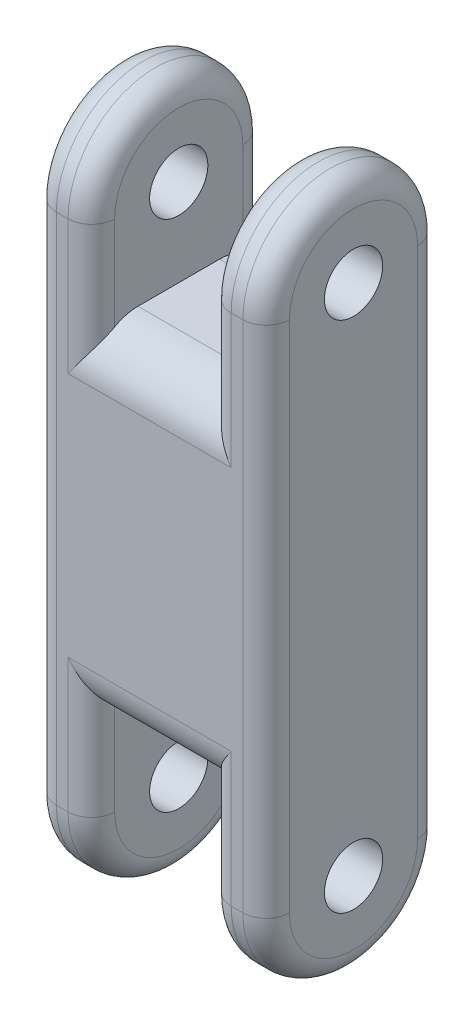
SolidWorks part; units mm, degrees
material "ABS"
ref_plane "Front" through (0, 0, 0) normal (0, 0, 1) x (1, 0, 0)
ref_plane "Top" through (0, 0, 0) normal (0, 1, 0) x (1, 0, 0)
ref_plane "Right" through (0, 0, 0) normal (1, 0, 0) x (0, 0, -1)
sketch "Sketch1" plane through (0, 0, 0) normal (1, 0, 0) x (0, 0, -1)
  line L0 (-4.7625, 0) -> (-4.7625, 27.9908)
  line L1 (4.7625, 27.9908) -> (4.7625, 0)
  arc A0 (-4.7625, 27.9908) -> (4.7625, 27.9908) centre (0, 27.9908) cw
  arc A1 (4.7625, 0) -> (-4.7625, 0) centre (0, 0) cw
  dimension "D1" = 9.525
  dimension "D2" = 27.9908
extrude "Boss-Extrude1" add sketch "Sketch1" along normal blind 12.7
sketch "Sketch2" plane through (12.7, 0, 0) normal (1, 0, 0) x (0, 0, -1)
  circle A0 centre (0, 0) radius 1.5875
  circle A1 centre (0, 27.9908) radius 1.5875
  dimension "D1" = 3.175
extrude "Cut-Extrude1" cut sketch "Sketch2" against normal blind 19.05
sketch3d "3DSketch1"
  line L0 (6.35, 27.9908, -4.7625) -> (6.35, 23.2283, -4.7625)
  line L1 (12.7, 27.9908, -4.7625) -> (0, 27.9908, -4.7625) construction
  line L2 (12.7, 27.9908, 4.7625) -> (0, 27.9908, 4.7625) construction
  line L3 (6.35, 27.9908, 4.7625) -> (6.35, 23.2283, 4.7625)
  line L5 (6.35, 0, 4.7625) -> (6.35, 4.7625, 4.7625)
  line L7 (12.7, 0, 4.7625) -> (0, 0, 4.7625) construction
  line L8 (12.7, 0, -4.7625) -> (0, 0, -4.7625) construction
  line L9 (6.35, 0, -4.7625) -> (6.35, 4.7625, -4.7625)
  line L10 (6.35, 23.2283, -4.7625) -> (6.35, 23.2283, 4.7625)
  line L11 (6.35, 4.7625, -4.7625) -> (6.35, 4.7625, 4.7625)
  arc A0 (6.35, 27.9908, -4.7625) -> (6.35, 27.9908, 4.7625) centre (6.35, 27.9908, 0) ccw
  arc A2 (6.35, 0, 4.7625) -> (6.35, 0, -4.7625) centre (6.35, 0, 0) ccw
  point P6 (11.1125, 27.9908, 0)
  point P18 (11.1125, 0, 0)
  dimension "D1" = 4.7625
  dimension "D2" = 4.7625
extrude "Cut-Extrude2" cut sketch "3DSketch1" along direction (-1, 0, 0) on the side against the normal mid plane 6.35
fillet "Fillet2" radius 2.54 4 edges
fillet "Fillet3" radius 1.27 20 edges at (0, 32.7533, 0) (0, 13.9954, -4.7625) (0, -4.7625, 0) (12.7, 32.7533, 0) (12.7, 13.9954, -4.7625) (12.7, -4.7625, 0) (0, 13.9954, 4.7625) (12.7, 13.9954, 4.7625)
sketch "Sketch3" plane through (0, 0, 0) normal (-1, 0, 0) x (0, 0, 1)
  line L0 (-3.4925, 27.9908) -> (-3.4925, 0) construction
  circle A0 centre (-2.2257, 2.096) radius 1.0868
  arc A2 (-3.4925, 0) -> (3.4925, 0) centre (0, 0) ccw construction
  dimension "D1" = 2.1736
  dimension "D2" = 1.2668
  dimension "D3" = 3.0573
extrude "Boss-Extrude2" add sketch "Sketch3" along normal blind 2.54
fillet "Fillet4" radius 0.762 1 edges at (-2.54, 2.096, -1.1389)
ref_plane "Plane1" through (0, 3.477, -2.0074) normal (0, 0.866, -0.5) x (-1, 0, 0)
sketch "Sketch4" plane through (0, 3.477, -2.0074) normal (0, 0.866, -0.5) x (-1, 0, 0)
  line L0 (0, 10.9708) -> (0, -3.0246) construction
  line L3 (-1.905, -4.1244) -> (-1.27, -4.1244) construction
  circle A0 centre (0.8566, -0.8068) radius 0.4916
  dimension "D1" = 0.8566
  dimension "D2" = 3.3177
  dimension "D3" = 0.9831
extrude "Cut-Extrude3" cut sketch "Sketch4" against normal blind 2.54
scale "Scale ratio 1" scale about origin uniform scaling yes scale factor 1.3
